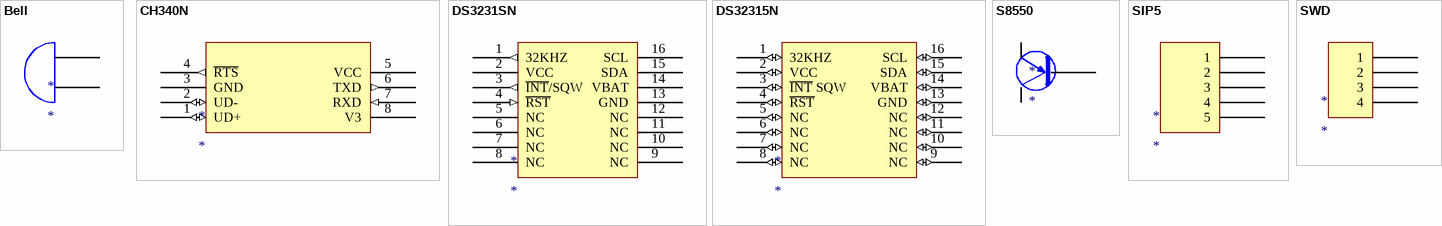
[diagram p0: symbols Bell to SWD]
# Altium schematic symbol library MISC82121-10.SchLib: 7 symbols
Pins are listed as number, name and electrical type; pins without a type are passive.


## Bell
designator *
pins: B16, B17

## CH340N
designator *
pins: 1 UD+ (io), 2 UD- (io), 3 GND, 4 ~{RTS} (out), 5 VCC, 6 TXD (out), 7 RXD (in), 8 V3

## DS3231SN
designator *
pins: 1 32KHZ (out), 2 VCC, 3 ~{INT}/SQW (out), 4 ~{RST} (in), 5 NC, 6 NC, 7 NC, 8 NC, 9 NC, 10 NC, 11 NC, 12 NC, 13 GND, 14 VBAT, 15 SDA, 16 SCL

## DS32315N
designator *
pins: 1 32KHZ (io), 2 VCC (io), 3 ~{INT} SQW (io), 4 ~{RST} (io), 5 NC (io), 6 NC (io), 7 NC (io), 8 NC (io), 9 NC (io), 10 NC (io), 11 NC (io), 12 NC (io), 13 GND (io), 14 VBAT (io), 15 SDA (io), 16 SCL (io)

## S8550
designator *
pins: B19, B20, B21

## SIP5
designator *
pins: B24 5, B25 4, B26 3, B27 2, B28 1

## SWD
designator *
pins: 1, 2, 3, 4